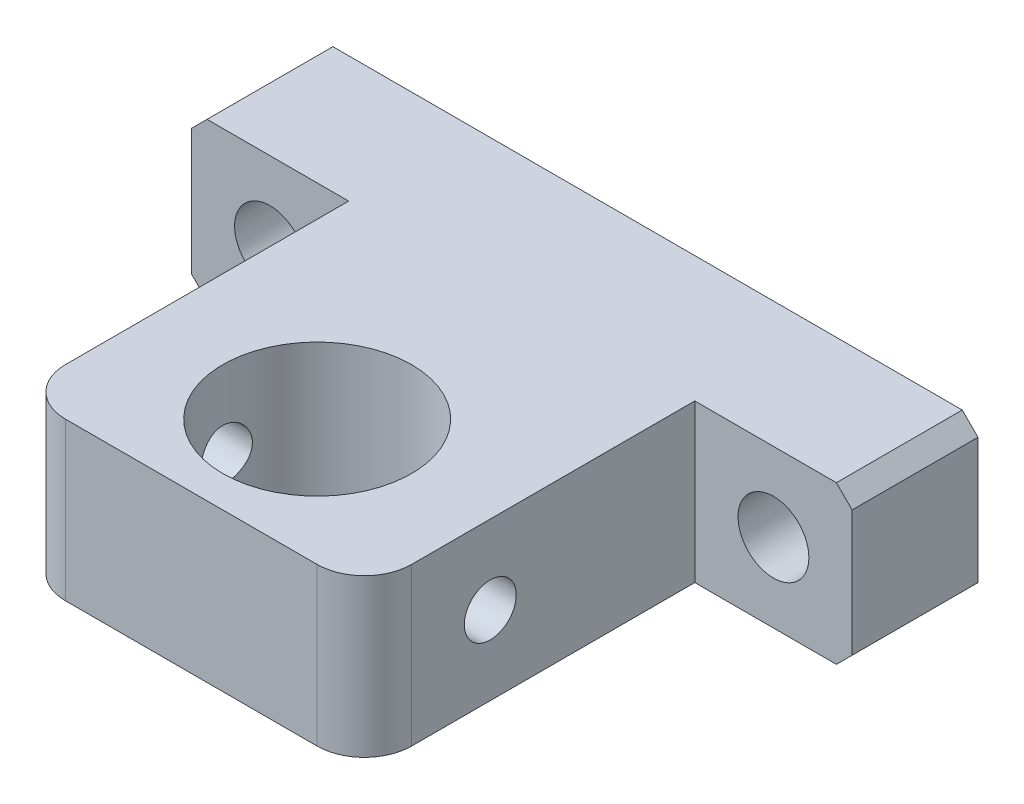
SolidWorks part; units mm, degrees
ref_plane "前视基准面" through (0, 0, 0) normal (0, 0, 1) x (1, 0, 0)
ref_plane "上视基准面" through (0, 0, 0) normal (0, 1, 0) x (1, 0, 0)
ref_plane "右视基准面" through (0, 0, 0) normal (1, 0, 0) x (0, 0, -1)
sketch "草图1" plane through (0, 0, 0) normal (0, 0, 1) x (1, 0, 0)
  line L1 (-21, 5) -> (21, 5)
  line L2 (-21, 5) -> (-21, -5)
  line L3 (-21, -5) -> (21, -5)
  line L4 (21, 5) -> (21, -5)
  line L5 (-21, 5) -> (21, -5) construction
  line L6 (-21, -5) -> (21, 5) construction
  point P0 (0, 0)
  dimension "D1" = 42
  dimension "D2" = 10
extrude "凸台-拉伸1" add sketch "草图1" along normal blind 8
sketch "草图2" plane through (0, 0, 8) normal (0, 0, 1) x (1, 0, 0)
  line L1 (-11, 5) -> (11, 5)
  line L2 (-11, 5) -> (-11, -5)
  line L3 (-11, -5) -> (11, -5)
  line L4 (11, 5) -> (11, -5)
  line L5 (-11, 5) -> (11, -5) construction
  line L6 (-11, -5) -> (11, 5) construction
  point P0 (0, 0)
  dimension "D1" = 22
  dimension "D2" = 10
extrude "凸台-拉伸2" add sketch "草图2" along normal offset from surface (21 mm away) 29 up to face at (0, 0, 0)
sketch "草图3" plane through (0, 5, 0) normal (0, 1, 0) x (1, 0, 0)
  line L0 (21, 0) -> (-21, 0) construction
  circle A0 centre (0, -21) radius 6
  dimension "D2" = 12
  dimension "D1" = 21
extrude "切除-拉伸1" cut sketch "草图3" against normal through all
sketch "草图4" plane through (0, 5, 0) normal (0, 1, 0) x (1, 0, 0)
  line L0 (11, -11) -> (5, -11)
  line L1 (11, -29) -> (11, -8) construction
  line L2 (5, -11) -> (5, -21)
  line L3 (5, -21) -> (6, -21)
  line L4 (6, -21) -> (6, -12)
  line L5 (6, -12) -> (11, -12)
  line L6 (11, -12) -> (11, -11)
  line L7 (21, 0) -> (-21, 0) construction
  circle A1 centre (0, -21) radius 6 construction
  dimension "D1" = 1
  dimension "D2" = 11
  dimension "D3" = 1
extrude "切除-拉伸2" [suppressed] cut sketch "草图4" against normal through all
fillet "圆角1" [suppressed] radius 6.5
hole_wizard "Ø4.5 (4.5) 直径孔1" positions "草图6" profile "草图5" hole size "Ø4.5" standard "GB"
sketch "草图6" [suppressed] plane through (0, 0, 5) normal (0, 0, 1) x (1, 0, 0)
  line L0 (0, -5) -> (0, 5) construction
  point P0 (-15, 0)
  point P2 (15, 0)
  dimension "D1" = 15
  dimension "D2" = 15
sketch "草图5" plane through (-15, 0, 5) normal (1, 0, 0) x (0, -1, 0)
  line L0 (0, 0) -> (0, 5)
  line L1 (0, 5) -> (2.25, 5)
  line L2 (2.25, 5) -> (2.25, 0)
  line L5 (2.25, 0) -> (0, 0)
  line L11 (0, -6.35) -> (0, 107.95) construction
  dimension "通孔孔直径" = 4.5
  dimension "通孔孔深度" = 5
hole_wizard "Ø4.5 (4.5) 直径孔2" positions "草图8" profile "草图7" hole size "Ø4.5" standard "GB" end condition through all
sketch "草图8" plane through (0, 0, 8) normal (0, 0, 1) x (1, 0, 0)
  point P0 (-16, 0)
  point P2 (16, 0)
  dimension "D1" = 16
  dimension "D2" = 16
sketch "草图7" plane through (-16, 0, 8) normal (1, 0, 0) x (0, -1, 0)
  line L0 (0, 0) -> (0, 8)
  line L1 (0, 8) -> (2.25, 8)
  line L2 (2.25, 8) -> (2.25, 0)
  line L5 (2.25, 0) -> (0, 0)
  line L11 (0, -6.35) -> (0, 107.95) construction
  dimension "通孔孔直径" = 4.5
  dimension "通孔孔深度" = 8
hole_wizard "M4 螺纹孔1" positions "草图10" profile "草图9" tap size "M4" standard "GB" end condition through all
sketch "草图10" plane through (11, 0, 0) normal (1, 0, 0) x (0, 0, -1)
  line L0 (-29, 5) -> (-8, 5) construction
  line L1 (-29, -5) -> (-29, 5) construction
  point P0 (-21, 0)
  dimension "D1" = 5
  dimension "D2" = 8
sketch "草图9" plane through (11, 0, 21) normal (0, 1, 0) x (0, 0, -1)
  line L0 (0, 0) -> (0, 32)
  line L1 (0, 32) -> (1.65, 32)
  line L2 (1.65, 32) -> (1.65, 0)
  line L5 (1.65, 0) -> (0, 0)
  line L11 (0, -6.35) -> (0, 107.95) construction
  dimension "通孔螺纹孔钻头直径" = 3.3
  dimension "通孔螺纹孔钻头深度" = 32
cosmetic thread "孔螺蚊线1" parameters "D2"=4
fillet "圆角3" radius 3 2 edges at (-11, 0, 29) (11, 0, 29)
chamfer "倒角1" distance 1 angle 45 4 edges at (21, -5, 4) (21, 5, 4) (-21, -5, 4) (-21, 5, 4)
